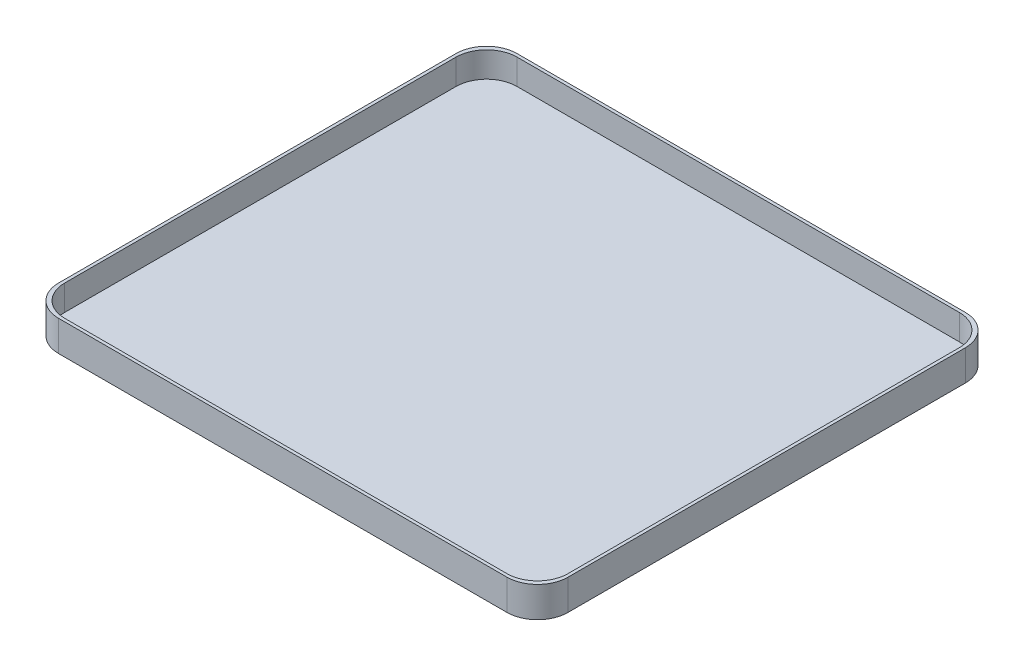
SolidWorks part; units mm, degrees
ref_plane "Front Plane" through (0, 0, 0) normal (0, 0, 1) x (1, 0, 0)
ref_plane "Top Plane" through (0, 0, 0) normal (0, 1, 0) x (1, 0, 0)
ref_plane "Right Plane" through (0, 0, 0) normal (1, 0, 0) x (0, 0, -1)
other "Configuration Table"
sketch "Sketch1" plane through (0, 0, 0) normal (0, 1, 0) x (1, 0, 0)
  line L1 (-220, 225) -> (220, 225)
  line L2 (-250, 195) -> (-250, -195)
  line L3 (-220, -225) -> (220, -225)
  line L4 (250, 195) -> (250, -195)
  line L5 (-250, 225) -> (250, -225) construction
  line L6 (-250, -225) -> (250, 225) construction
  arc A0 (-220, -225) -> (-250, -195) centre (-220, -195) cw
  arc A1 (250, -195) -> (220, -225) centre (220, -195) cw
  arc A2 (250, 195) -> (220, 225) centre (220, 195) ccw
  arc A3 (-220, 225) -> (-250, 195) centre (-220, 195) ccw
  point P0 (0, 0)
  dimension "D3" = 30
  dimension "D1" = 500
  dimension "D2" = 450
extrude "Boss-Extrude1" add sketch "Sketch1" along normal blind 30
sketch "Sketch2" plane through (0, 30, 0) normal (0, 1, 0) x (1, 0, 0)
  line L1 (-217, 222) -> (217, 222)
  line L2 (-247, 192) -> (-247, -192)
  line L3 (-217, -222) -> (217, -222)
  line L4 (247, 192) -> (247, -192)
  line L5 (-247, 222) -> (247, -222) construction
  line L6 (-247, -222) -> (247, 222) construction
  arc A0 (217, -222) -> (247, -192) centre (217, -192) ccw
  arc A1 (247, 192) -> (217, 222) centre (217, 192) ccw
  arc A2 (-247, 192) -> (-217, 222) centre (-217, 192) cw
  arc A3 (-247, -192) -> (-217, -222) centre (-217, -192) ccw
  point P0 (0, 0)
  dimension "D3" = 30
  dimension "D1" = 494
  dimension "D2" = 444
extrude "Cut-Extrude1" cut sketch "Sketch2" against normal blind 25
